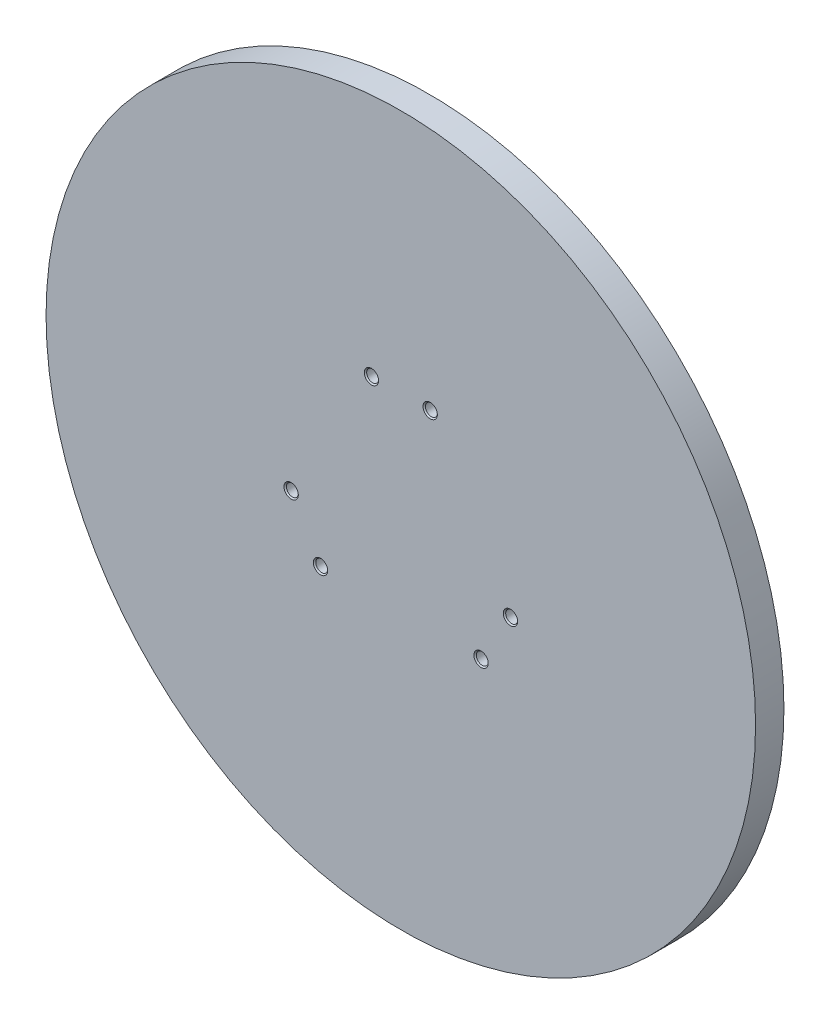
from build123d import *

# Parameters (mm, degrees)
SKETCH_1_R               = 125
EXTRUDE_1_DEPTH          = 10
M5X0_8_1_AT_2_COUNT      = 2
M5X0_8_1_AT_2_PITCH      = 20.705523608
PATTERN_CIRCULAR_1_COUNT = 3


with BuildPart() as part:
    # 草图1 → 凸台-拉伸1 (new body)
    with BuildSketch(Plane.XY):
        Circle(SKETCH_1_R)
    extrude(amount=EXTRUDE_1_DEPTH)

    # 草图4 → M5x0.8 螺纹孔1 (revolve, cut)
    with BuildSketch(Plane(origin=(10.352761804, 38.637033052, 10), x_dir=(0, -1, 0), z_dir=(1, 0, 0))):
        Polygon((0, 0), (0, 13.6618073), (2.1, 12.4), (2.1, 0.425), (2.525, 0), align=None)
    m5x0_8_1 = revolve(axis=Axis((10.352761804, 38.637033052, 16.35), (0, 0, -1)), mode=Mode.SUBTRACT)

    # M5x0.8 螺纹孔1 at 2: M5x0.8 螺纹孔1 ×2
    with Locations(*[(-i * M5X0_8_1_AT_2_PITCH, 0, 0) for i in range(1, M5X0_8_1_AT_2_COUNT)]):
        add(m5x0_8_1, mode=Mode.SUBTRACT)

    # 阵列(圆周)1: M5x0.8 螺纹孔1 ×3 about axis
    pattern_circular_1_axis = Axis((0, 0, 0), (0, 0, 1))
    for i in range(1, PATTERN_CIRCULAR_1_COUNT):
        add(m5x0_8_1.rotate(pattern_circular_1_axis, i * 360 / PATTERN_CIRCULAR_1_COUNT), mode=Mode.SUBTRACT)

    # 阵列(圆周)1 copy 1 sketch → 阵列(圆周)1 copy 1 (revolve, cut)
    with BuildSketch(Plane(origin=(-28.284271247, -28.284271247, 10), x_dir=(0.8660254037844387, 0.4999999999999998, 0), z_dir=(-0.4999999999999998, 0.8660254037844387, 0))):
        Polygon((0, 0), (0, 13.6618073), (2.1, 12.4), (2.1, 0.425), (2.525, 0), align=None)
    revolve(axis=Axis((-28.284271247, -28.284271247, 16.35), (0, 0, -1)), mode=Mode.SUBTRACT)

    # 阵列(圆周)1 copy 2 sketch → 阵列(圆周)1 copy 2 (revolve, cut)
    with BuildSketch(Plane(origin=(38.637033052, -10.352761804, 10), x_dir=(-0.8660254037844384, 0.5000000000000004, 0), z_dir=(-0.5000000000000004, -0.8660254037844384, 0))):
        Polygon((0, 0), (0, 13.6618073), (2.1, 12.4), (2.1, 0.425), (2.525, 0), align=None)
    revolve(axis=Axis((38.637033052, -10.352761804, 16.35), (0, 0, -1)), mode=Mode.SUBTRACT)


solid = part.part
